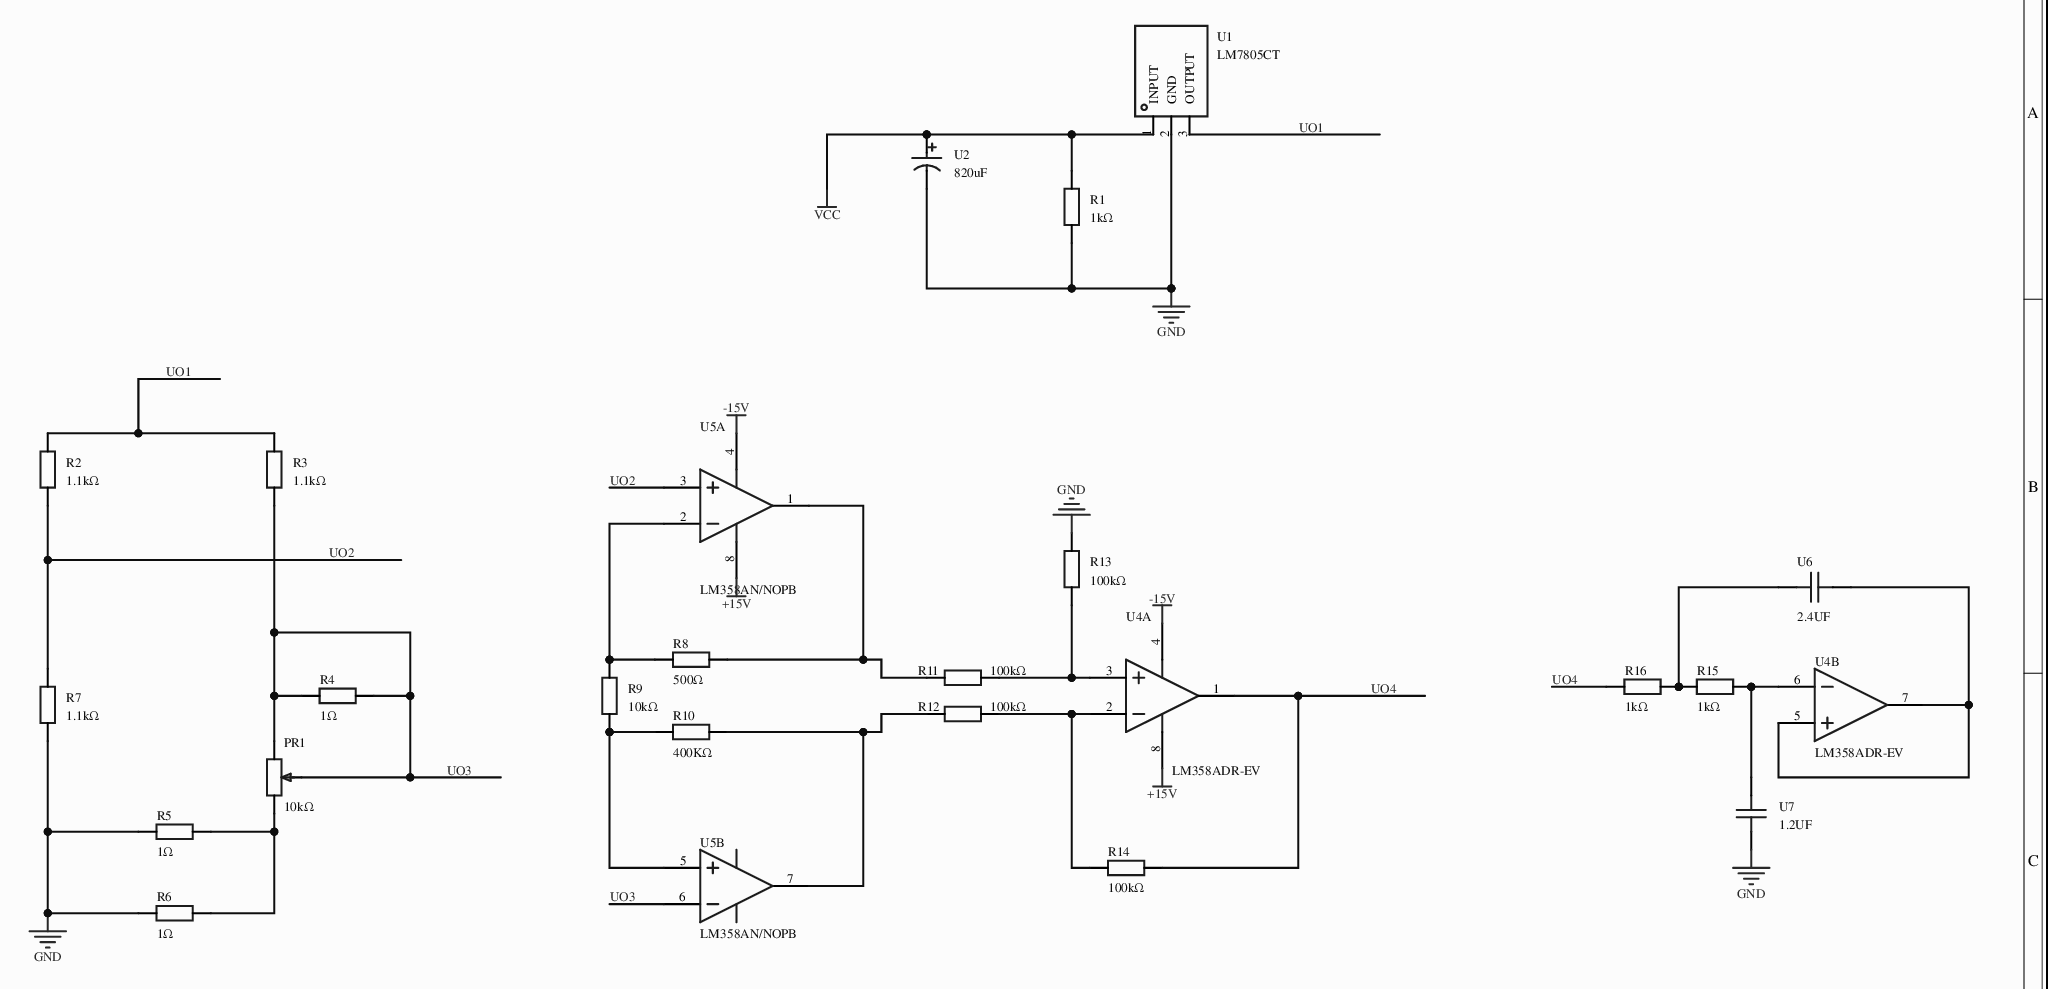
[diagram p0: MISC51804-3.schdoc]
# Altium project MISC51804-2.PrjPcb
1 sheet, 23 parts. Net scope: global (net labels, ports and power ports of the same name join across sheets).
Board file: MISC51804.pcbdoc

## Sheet MISC51804-3.schdoc
size 297 x 209 mm; Version: V1.0; @Project Name: MISC51804; @Update Date: 2026-04-20; @Create Date: 2026-04-20; @Board Name: MISC51804; @Create Time: 21:47:58; @Page Count: 1; @Page No: 1; @Schematic Name: MISC51804; @Update Time: 21:47:58; Size: A4

### Parts
PR1  10kΩ  [R_3296]
R1  1kΩ  [Res_1/8W]
R2  1.1kΩ  [Res_1/8W]
R3  1.1kΩ  [Res_1/8W]
R4  1Ω  [Res_1/8W]
R5  1Ω  [Res_1/8W]
R6  1Ω  [Res_1/8W]
R7  1.1kΩ  [Res_1/8W]
R8  500Ω  [Res_1/8W]
R9  10kΩ  [Res_1/8W]
R10  400KΩ  [Res_1/8W]
R11  100kΩ  [Res_1/8W]
R12  100kΩ  [Res_1/8W]
R13  100kΩ  [Res_1/8W]
R14  100kΩ  [Res_1/8W]
R15  1kΩ  [Res_1/8W]
R16  1kΩ  [Res_1/8W]
U1  LM7805CT  [TO-220-3_L10.0-W4.5-P2.54-L]
U2  820uF  [CAP-TH_BD22.0-P10.00-D2.2-FD]
U4  LM358ADR-EV  [SOIC-8_L4.9-W3.9-P1.27-LS6.0-BL]  (parts A,B of 2)
U5  LM358AN/NOPB  [PDIP-8_L10.2-W6.5-P2.54-LS7.6-BL]  (parts A,B of 2)
U6  2.4UF  [CAP-TH_L5.0-W2.5-P5.00-D1.0]
U7  1.2UF  [CAP-TH_L5.0-W2.5-P5.00-D1.0]

### Nets
+15V: U4.8(V+) U5.8(V+)
-15V: U4.4(V-) U5.4(GND)
GND: R1.1 R5.2 R6.2 R7.1 R13.2 U1.2(GND) U2.2 U7.2
VCC: R1.2 U1.1(INPUT) U2.1
UO1: R2.2 R3.2 U1.3(OUTPUT)
UO2: R2.1 R7.2 U5.3(INA+)
UO3: PR1.2 PR1.3 R3.1 R4.1 R4.2 U5.6(INB-)
UO4: R14.1 R16.1 U4.1(OUT1)
NetPR1_1: PR1.1 R5.1 R6.1
NetR8_1: R8.1 R9.2 U5.2(INA-)
NetR8_2: R8.2 R11.1 U5.1(OUTA)
NetR9_1: R9.1 R10.1 U5.5(INB+)
NetR10_2: R10.2 R12.1 U5.7(OUTB)
NetR11_2: R11.2 R13.1 U4.3(IN1+)
NetR12_2: R12.2 R14.2 U4.2(IN1-)
NetR15_1: R15.1 R16.2 U6.2
NetR15_2: R15.2 U4.6(IN2-) U7.1
NetU4_5: U4.5(IN2+) U4.7(OUT2) U6.1

### Library data of the parts
PR1 = R_3296: ConvertToPcb: yes; ModelId: b182808559bb43bda9e7de64b64134cb0819f05c4eef4c71ace90d822a990e87; ModelName: 3296W; ModelTransform: 373.98,188.96,590.49,180,0,0,0,0,-140; Symbol: R_3296; Device: R_3296; AddInBom: yes; Supplier Footprint: 直插; FootprintName: R_3296; Value: 10kΩ
R1-R16 = Res_AXIAL-1/8W: Symbol: 电阻; ConvertToPcb: yes; ModelId: b2b5ae7ae4c642178fe0039925c86a3f0819f05c4eef4c71ace90d822a990e87; ModelName: RES-TH_BD1.8-L3.2-P7.20-D0.4; ModelTransform: 282.86,66.88,253.09,0,0,0,0,0,-191; Device: Res_AXIAL-1/8W; AddInBom: yes; Supplier Footprint: 轴向引线; FootprintName: Res_1/8W
  R1 R15 R16: Value: 1kΩ
  R2 R3 R7: Value: 1.1kΩ
  R4-R6: Value: 1Ω
  R8: Value: 500Ω
  R9: Value: 10kΩ
  R10: Value: 400KΩ
  R11-R14: Value: 100kΩ
U1 = LM7805CT: 输出类型:固定;工作电压:35V;输出电压:5V;输出电流:1.5A;电源纹波抑制比(PSRR):62dB@(120Hz);输出极性:正极;; Manufacturer: HGSEMI(华冠); Symbol: LM7805CT_C725349; AddInBom: yes; ModelId: b3c9e38e4428458f8b925050989b538f0819f05c4eef4c71ace90d822a990e87; ModelTransform: 401.574,178.58232,0,0,0,0,0,25.59,-196.85; Output Type: 固定; Voltage - Supply: 35V; Output Voltage: 5V; Output Current: 1.5A; Voltage Dropout: 2V@(1A); standby current: 8mA; Noise: 40uV; Output Configuration: 正极; Number of Outputs: 1; Device: LM7805CT; LCSC Part Name: 1A 宽输入电压固定电压稳压器; SupplierPart: C725349; ManufacturerPart: LM7805CT; Supplier Footprint: TO-220; JLCPCB Part Class: Extended Part; Datasheet: https://item.szlcsc.com/datasheet/LM7805CT/771583.html; Supplier: LCSC; ConvertToPcb: yes; FootprintName: TO-220-3_L10.0-W4.5-P2.54-L; ModelName: TO-220-3_L10.0-W4.5-P2.54-L; Power Supply Rejection Ratio (PSRR): 62dB@(120Hz); Features: 短路保护；过热保护; Operating Temperature: -55℃~+150℃@(Tj)
U2 = LGG2D821MELZ40: 容值:820uF;精度:±20%;额定电压:200V;脚间距:10mm;等效串联电阻:-;纹波电流:1.75A@120Hz;; Manufacturer: Nichicon(尼吉康); AddInBom: yes; ModelId: f93741c73fcc4f4bb77f9d80a9a96aee0819f05c4eef4c71ace90d822a990e87; ModelTransform: 866.14,866.14,0,325,0,0,0,-0.039,-196.85; Tolerance: ±20%; Rated Voltage: 200V; φD: 22mm; L: 40mm; Lifetime @ Temperature: 2000hrs@105℃; Symbol: LGG2D821MELZ40; Device: LGG2D821MELZ40; LCSC Part Name: 820uF ±20% 200V; SupplierPart: C1581370; ManufacturerPart: LGG2D821MELZ40; Supplier Footprint: 插件,D22xL40mm; JLCPCB Part Class: Extended Part; Datasheet: https://atta.szlcsc.com/upload/public/pdf/source/20211019/0780858BB22DE4DB3764512238AA97AB.pdf; Supplier: LCSC; ConvertToPcb: yes; FootprintName: CAP-TH_BD22.0-P10.00-D2.2-FD; ModelName: CAP-TH_BD22.0-P10.00-D2.2-FD; Value: 820uF; Lead Spacing: 10mm; Equivalent Series Resistance (ESR): -; Ripple Current: 1.75A@120Hz; Operating Temperature: -40℃~+105℃
U4 = LM358ADR-EV: 放大器数:双路;输入失调电压(Vos):2mV;输入偏置电流(Ib):40nA;; Relevance: []; AddInBom: yes; ModelId: e81d2f7d937b4a6ab1dca543ff5d56a40819f05c4eef4c71ace90d822a990e87; ModelName: SOIC-8_L4.9-W3.9-H1.7-LS6.0-P1.27; ModelTransform: 192.913,236.22,0,0,0,0,0,0,0; Number of Circuits: 双路; Voltage - Input Offset(Vos): 2mV; Current - Input Bias(Ib): 40nA; Symbol: LM358ADR-EV; Device: LM358ADR-EV; LCSC Part Name: LM358ADR-EV; SupplierPart: C28642199; ManufacturerPart: LM358ADR-EV; Supplier Footprint: SOP-8; JLCPCB Part Class: Extended Part; Datasheet: https://atta.szlcsc.com/upload/public/pdf/source/20240712/81EA77249C59C376F31EAEA0E38D44C6.pdf; Supplier: LCSC; ConvertToPcb: yes; FootprintName: SOIC-8_L4.9-W3.9-P1.27-LS6.0-BL
U5 = LM358AN/NOPB: 放大器数:2;轨到轨:-;增益带宽积(GBW):1MHz;输入失调电压(Vos):2mV;压摆率(SR):-;输入偏置电流(Ib):50nA;; Manufacturer: TI(德州仪器); Relevance: []; AddInBom: yes; ModelId: b5bb019b7dad497cba3f645155e53c260819f05c4eef4c71ace90d822a990e87; ModelTransform: 401.574,311.8104,0,0,0,0,0,0,-137.795; Number of Channels: 2; Maximum Power Supply Range (Vdd-Vss): 32V; Gain Bandwidth Product: 1MHz; Vos - Input Offset Voltage: 2mV; Input Offset Voltage Drift(Vos TC): 7uV/℃; Ib - Input Bias Current: 50nA; Common Mode Rejection Ratio(CMRR): 85dB; Quiescent Current: 500uA; Output Current: 40mA; Single supply: 3V~32V; Dual Supply: -16V~-1.5V；1.5V~16V; Symbol: LM358AN/NOPB; Device: LM358AN/NOPB; LCSC Part Name: LM358AN/NOPB; SupplierPart: C1348620; ManufacturerPart: LM358AN/NOPB; Supplier Footprint: PDIP-8; JLCPCB Part Class: Extended Part; Datasheet: https://www.ti.com/cn/lit/gpn/lm158-n; Supplier: LCSC; ConvertToPcb: yes; FootprintName: PDIP-8_L10.2-W6.5-P2.54-LS7.6-BL; ModelName: PDIP-8_L10.2-W6.5-P2.54-LS7.6-BL; Rail to Rail: -; Slew Rate: -; Input Offset Current(Ios): 50nA; Input Voltage Noise Density: -; Input offset current drift(Ios TC): -; Operating Temperature: 0℃~+70℃
U6 U7 = 100nF: Symbol: 100NF_C9900015256; AddInBom: yes; ModelId: 08e3d7481fc7486bb1b263873f51e1e10819f05c4eef4c71ace90d822a990e87; ModelName: CAP-TH_BD5.0-W2.5-P5.08; ModelTransform: 224.652,98.425,0,0,0,0,-0.005,0,-137.795; Device: 100nF; LCSC Part Name: 100nF; SupplierPart: C9900015256; Supplier Footprint: CAP-TH_L5.0-W2.5-P5.00-D1.0; JLCPCB Part Class: Extended Part; Supplier: LCSC; ConvertToPcb: yes; FootprintName: CAP-TH_L5.0-W2.5-P5.00-D1.0
  U6: Manufacturer Part: 2.4UF
  U7: Manufacturer Part: 1.2UF